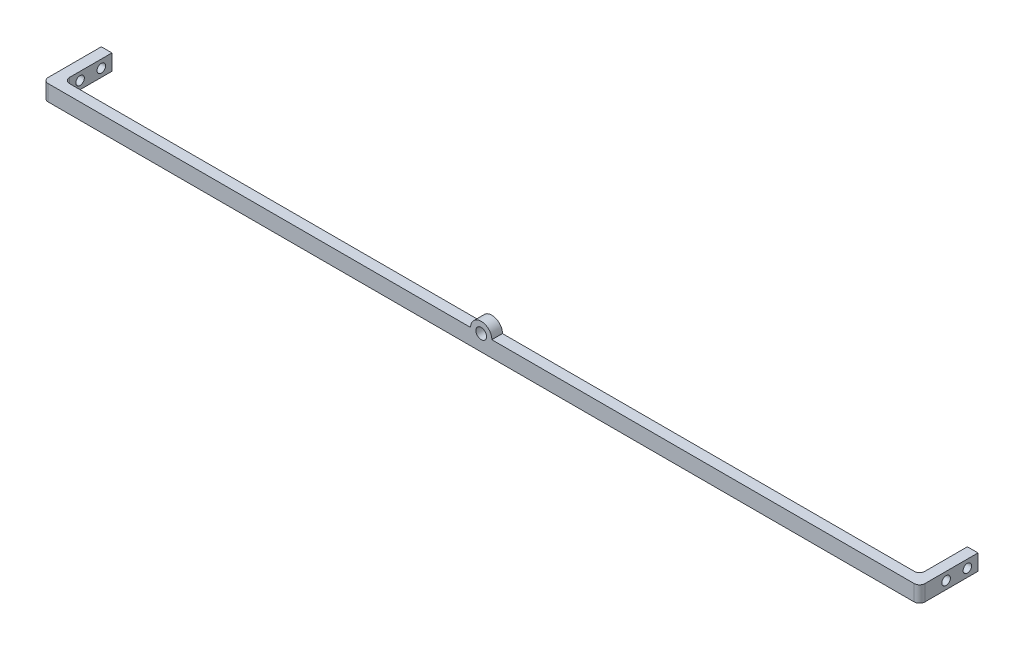
SolidWorks part; units mm, degrees
ref_plane "前视基准面" through (0, 0, 0) normal (0, 0, 1) x (1, 0, 0)
ref_plane "上视基准面" through (0, 0, 0) normal (0, 1, 0) x (1, 0, 0)
ref_plane "右视基准面" through (0, 0, 0) normal (1, 0, 0) x (0, 0, -1)
sketch "草图1" plane through (0, 0, 0) normal (0, 0, 1) x (1, 0, 0)
  line L1 (0, -15) -> (412.5, -15)
  line L2 (412.5, -15) -> (412.5, 0)
  line L4 (412.5, 0) -> (10, 0)
  line L5 (0, -15) -> (-412.5, -15)
  line L6 (-412.5, -15) -> (-412.5, 0)
  line L7 (-412.5, 0) -> (-10, 0)
  circle A0 centre (0, 0) radius 5
  arc A1 (10, 0) -> (-10, 0) centre (0, 0) ccw
extrude "凸台-拉伸1" add sketch "草图1" along normal blind 10
sketch "草图2" plane through (412.5, 0, 0) normal (1, 0, 0) x (0, 0, -1)
  line L1 (0, 0) -> (45, 0)
  line L2 (0, 0) -> (0, -15)
  line L3 (0, -15) -> (45, -15)
  line L4 (45, 0) -> (45, -15)
  circle A0 centre (15, -7.5) radius 4
  circle A1 centre (35, -7.5) radius 4
  dimension "D1" = 15
  dimension "D2" = 20
extrude "凸台-拉伸2" add sketch "草图2" against normal blind 10
sketch "草图3" plane through (-412.5, 0, 0) normal (-1, 0, 0) x (0, 0, 1)
  line L1 (0, 0) -> (-45, 0)
  line L2 (0, 0) -> (0, -15)
  line L3 (0, -15) -> (-45, -15)
  line L4 (-45, 0) -> (-45, -15)
  circle A0 centre (-35, -7.5) radius 4
  circle A1 centre (-15, -7.5) radius 4
extrude "凸台-拉伸3" add sketch "草图3" against normal blind 10
fillet "圆角1" radius 5 4 edges at (-412.5, -7.5, 10) (412.5, -7.5, 10) (-402.5, -7.5, 0)
